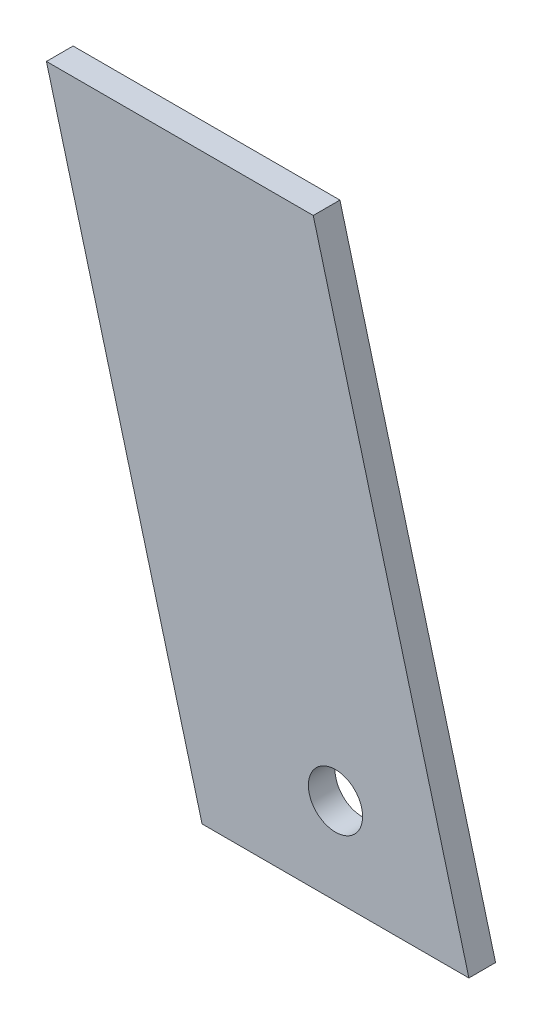
from build123d import *

# Parameters (mm, degrees)
EXTRUDE_1_DEPTH     = 3
SKETCH_2_R          = 6.1
CUT_EXTRUDE_1_DEPTH = 15


with BuildPart() as part:
    # 草图1 → 凸台-拉伸1 (new, symmetric)
    with BuildSketch(Plane.XY):
        Polygon((-30, -36), (30, -36), (65, -167), (5, -167), align=None)
    extrude(amount=EXTRUDE_1_DEPTH, both=True)

    # 草图2 → 切除-拉伸1 (cut, symmetric)
    with BuildSketch(Plane.XY):
        with Locations(Location((35, -147.5, 0), (0, 0, 180))):
            Circle(SKETCH_2_R)
    extrude(amount=CUT_EXTRUDE_1_DEPTH, both=True, mode=Mode.SUBTRACT)


solid = part.part
